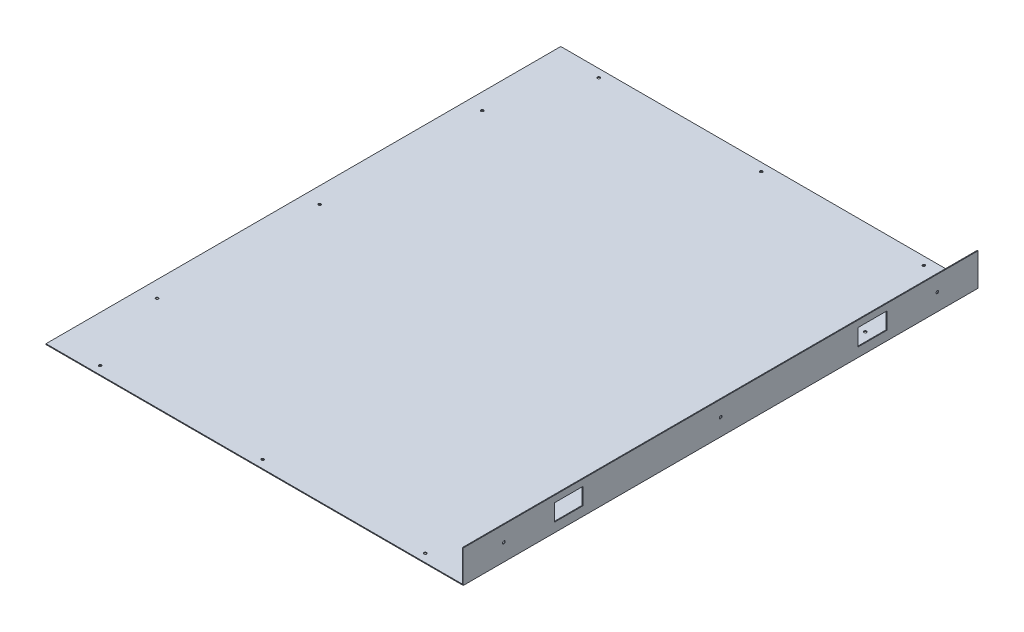
SolidWorks part; units mm, degrees
ref_plane "Front Plane" through (0, 0, 0) normal (0, 0, 1) x (1, 0, 0)
ref_plane "Top Plane" through (0, 0, 0) normal (0, 1, 0) x (1, 0, 0)
ref_plane "Right Plane" through (0, 0, 0) normal (1, 0, 0) x (0, 0, -1)
sketch "Sketch1" plane through (0, 0, 0) normal (0, 0, 1) x (1, 0, 0)
  line L0 (0, 0) -> (0, -60)
  line L1 (0, -60) -> (770, -60)
  line L2 (770, -60) -> (770, 0)
  line L3 (1.5, 0) -> (1.5, -58.5)
  line L4 (1.5, -58.5) -> (768.5, -58.5)
  line L5 (768.5, -58.5) -> (768.5, 0)
  line L6 (0, 0) -> (1.5, 0)
  line L7 (768.5, 0) -> (770, 0)
  dimension "D1" = 770
  dimension "D3" = 60
  dimension "D4" = 60
  dimension "D2" = 1.5
extrude "Boss-Extrude1" add sketch "Sketch1" along normal blind 950
sketch "Sketch2" plane through (770, 0, 0) normal (1, 0, 0) x (0, 0, -1)
  line L0 (0, -60) -> (0, 0) construction
  line L5 (-475, 0) -> (-475, 85.5947) construction
  line L6 (-729, -43) -> (-782, -12) construction
  line L7 (-221, -12) -> (-168, -12)
  line L8 (-221, -12) -> (-221, -43)
  line L9 (-221, -43) -> (-168, -43)
  line L10 (-168, -12) -> (-168, -43)
  line L11 (-221, -12) -> (-168, -43) construction
  line L12 (-221, -43) -> (-168, -12) construction
  line L13 (-950, 0) -> (0, 0) construction
  line L14 (-729, -12) -> (-782, -43) construction
  line L15 (-782, -12) -> (-782, -43)
  line L16 (-729, -43) -> (-782, -43)
  line L17 (-729, -12) -> (-729, -43)
  line L18 (-729, -12) -> (-782, -12)
  line L19 (-950, -60) -> (-950, 0) construction
  circle A0 centre (-75, -28.5) radius 2.5
  circle A1 centre (-475, -28.5) radius 2.5
  circle A2 centre (-875, -28.5) radius 2.5
  point P5 (-194.5, -27.5)
  point P15 (-755.5, -27.5)
  dimension "D7" = 5
  dimension "D9" = 5
  dimension "D1" = 53
  dimension "D2" = 31
  dimension "D3" = 168
  dimension "D4" = 12
  dimension "D5" = 28.5
  dimension "D6" = 75
  dimension "D8" = 75
extrude "Cut-Extrude1" cut sketch "Sketch2" against normal blind 1356.5
sketch "Sketch3" plane through (0, -60, 0) normal (0, -1, 0) x (1, 0, 0)
  line L0 (770, 950) -> (770, 0) construction
  line L1 (0, 950) -> (770, 950) construction
  line L2 (770, 475) -> (547.713, 475) construction
  circle A0 centre (737, 475) radius 2.5
  circle A1 centre (737, 775) radius 2.5
  circle A2 centre (737, 175) radius 2.5
  circle A3 centre (30, 775) radius 2.5
  circle A4 centre (30, 475) radius 2.5
  circle A5 centre (30, 175) radius 2.5
  circle A6 centre (385, 935) radius 2.5
  circle A7 centre (685, 935) radius 2.5
  circle A8 centre (85, 935) radius 2.5
  circle A9 centre (85, 15) radius 2.5
  circle A10 centre (685, 15) radius 2.5
  circle A11 centre (385, 15) radius 2.5
  point P9 (770, 475)
  point P25 (385, 950)
  dimension "D4" = 5
  dimension "D9" = 5
  dimension "D1" = 300
  dimension "D2" = 300
  dimension "D3" = 33
  dimension "D6" = 15
  dimension "D7" = 300
  dimension "D8" = 300
  dimension "D5" = 2
extrude "Cut-Extrude2" cut sketch "Sketch3" against normal blind 1.5
sketch "Sketch4" plane through (0, 0, 0) normal (0, 1, 0) x (1, 0, 0)
  line L4 (1.5, 0) -> (0, 0)
  line L5 (0, 0) -> (0, -950)
  line L6 (0, -950) -> (1.5, -950)
  line L7 (1.5, -950) -> (1.5, 0)
  line L8 (1.5, 0) -> (0, 0)
  line L9 (0, 0) -> (0, -950)
  line L10 (0, -950) -> (1.5, -950)
  line L11 (1.5, -950) -> (1.5, 0)
  dimension "D1" = 0
extrude "Cut-Extrude3" cut sketch "Sketch4" against normal up to surface (58.5 mm away) up to face at (85, -58.5, 17.5)
